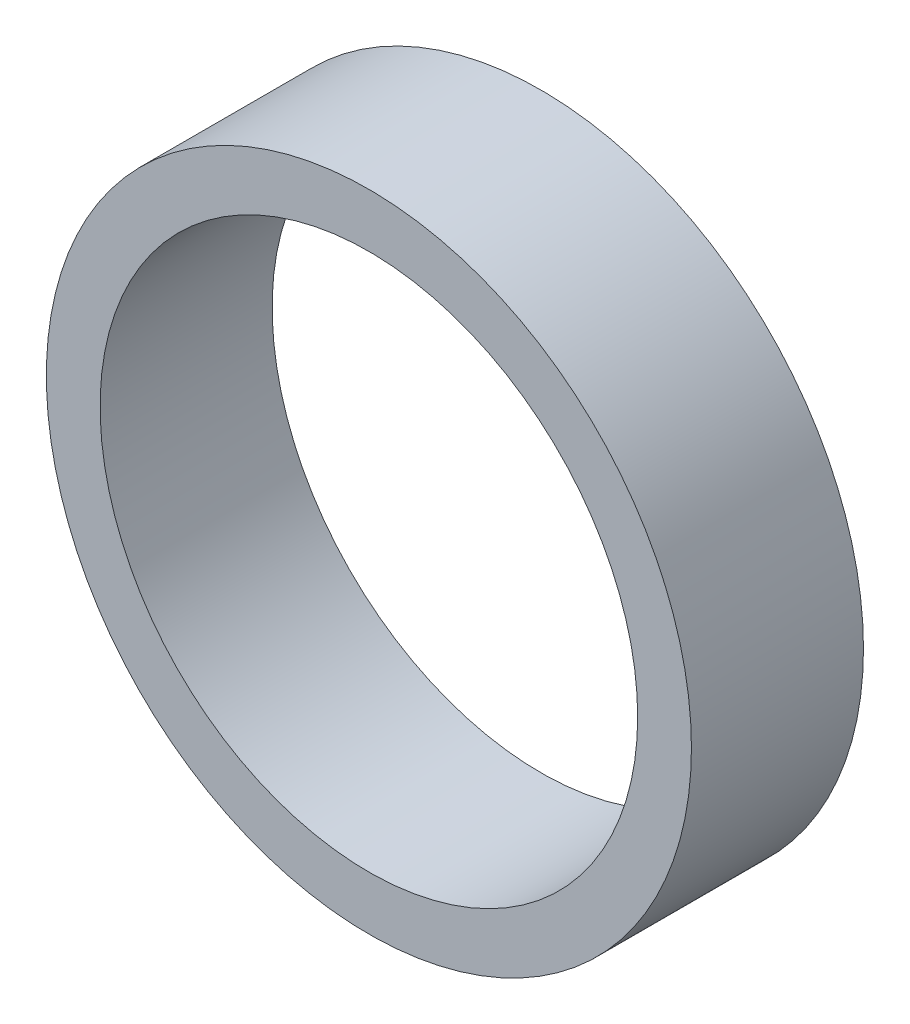
SolidWorks part; units mm, degrees
ref_plane "前视基准面" through (0, 0, 0) normal (0, 0, 1) x (1, 0, 0)
ref_plane "上视基准面" through (0, 0, 0) normal (0, 1, 0) x (1, 0, 0)
ref_plane "右视基准面" through (0, 0, 0) normal (1, 0, 0) x (0, 0, -1)
sketch "草图1" plane through (0, 0, 0) normal (0, 0, 1) x (1, 0, 0)
  circle A0 centre (0, 0) radius 12.5
  circle A1 centre (0, 0) radius 15
  dimension "D1" = 25
  dimension "D2" = 30
extrude "凸台-拉伸1" add sketch "草图1" along normal blind 8
